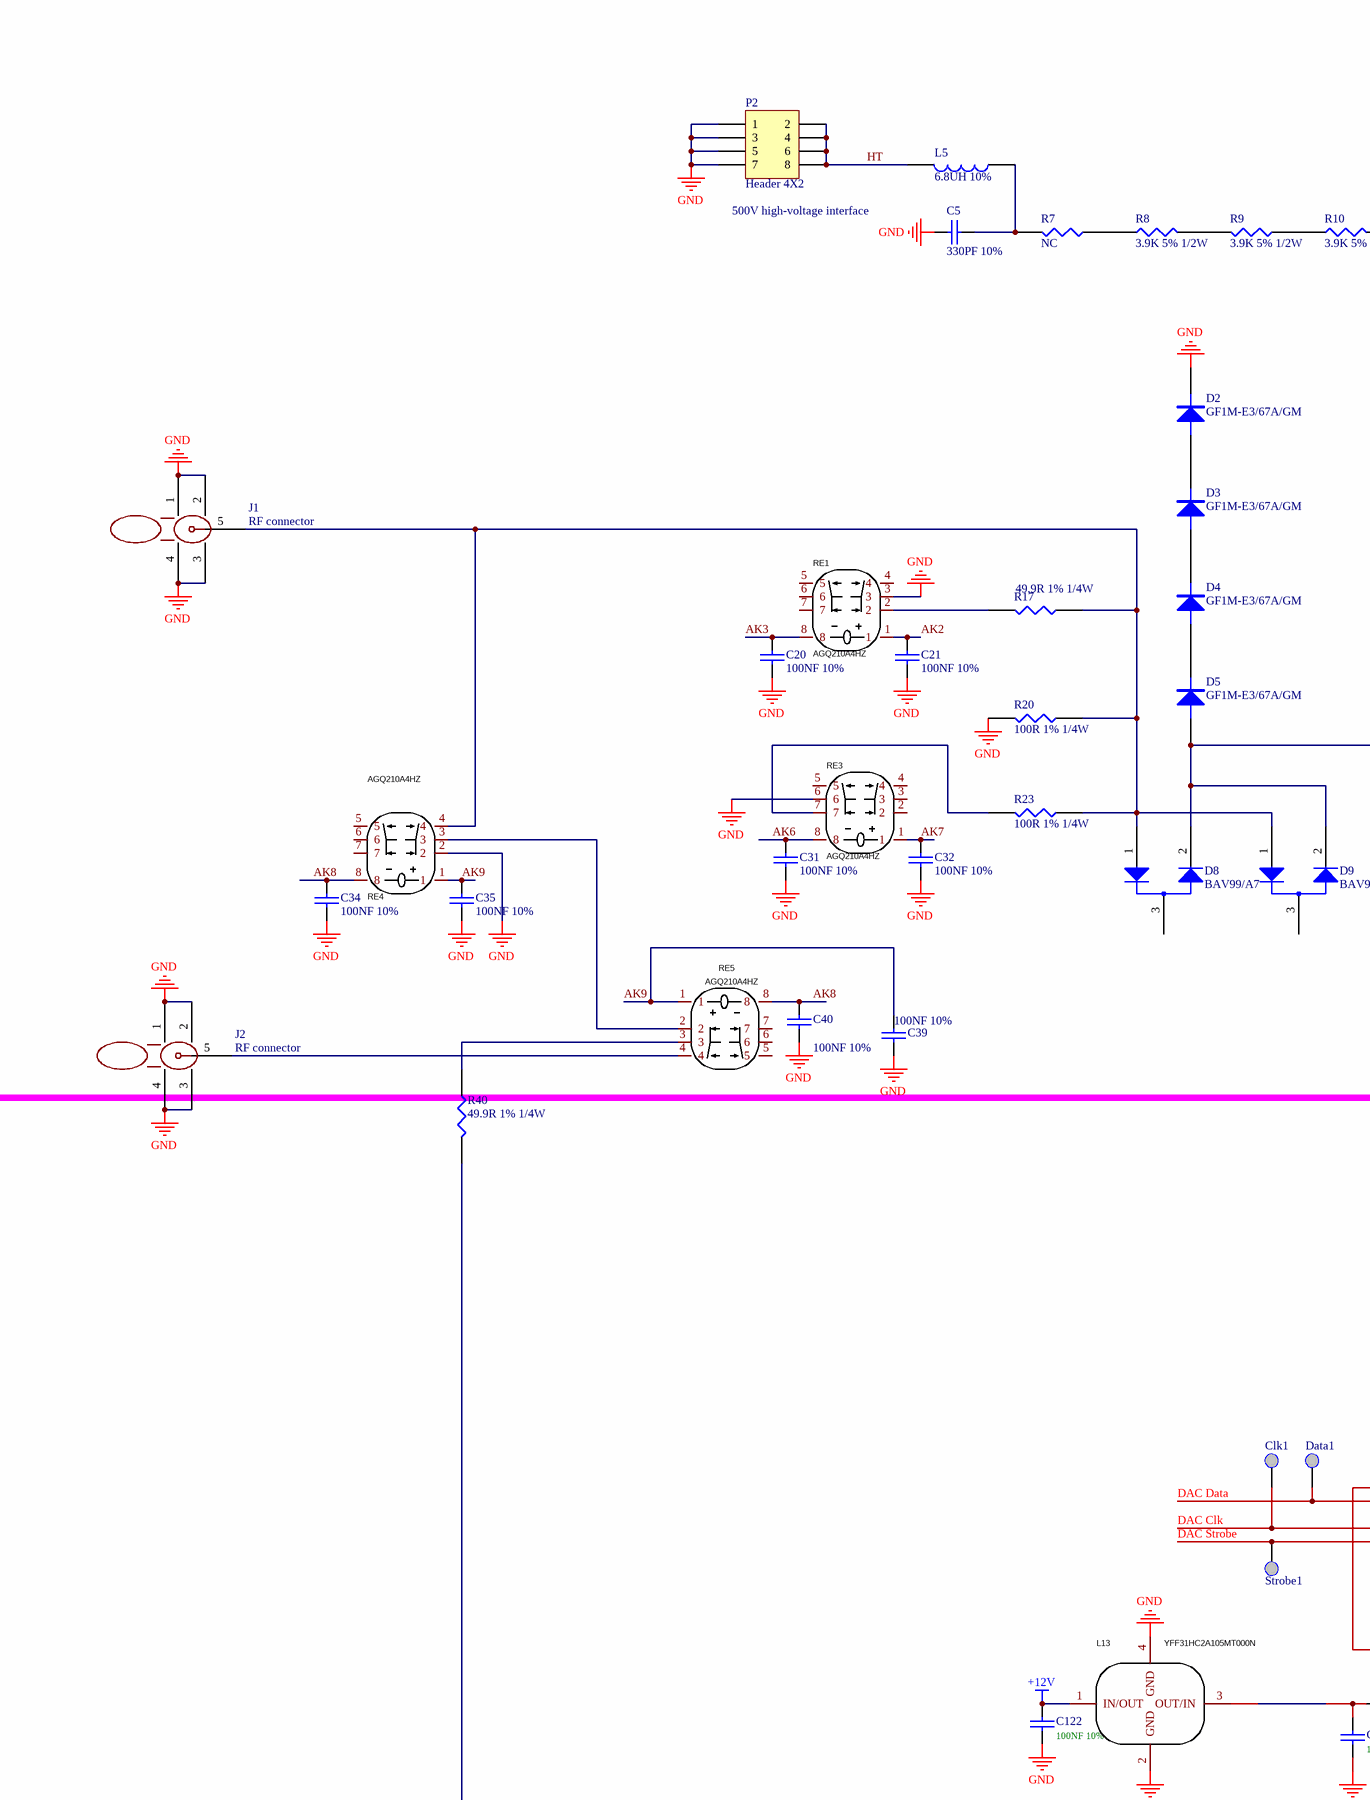
[diagram p0: PCBE109560-5.SchDoc, top left]
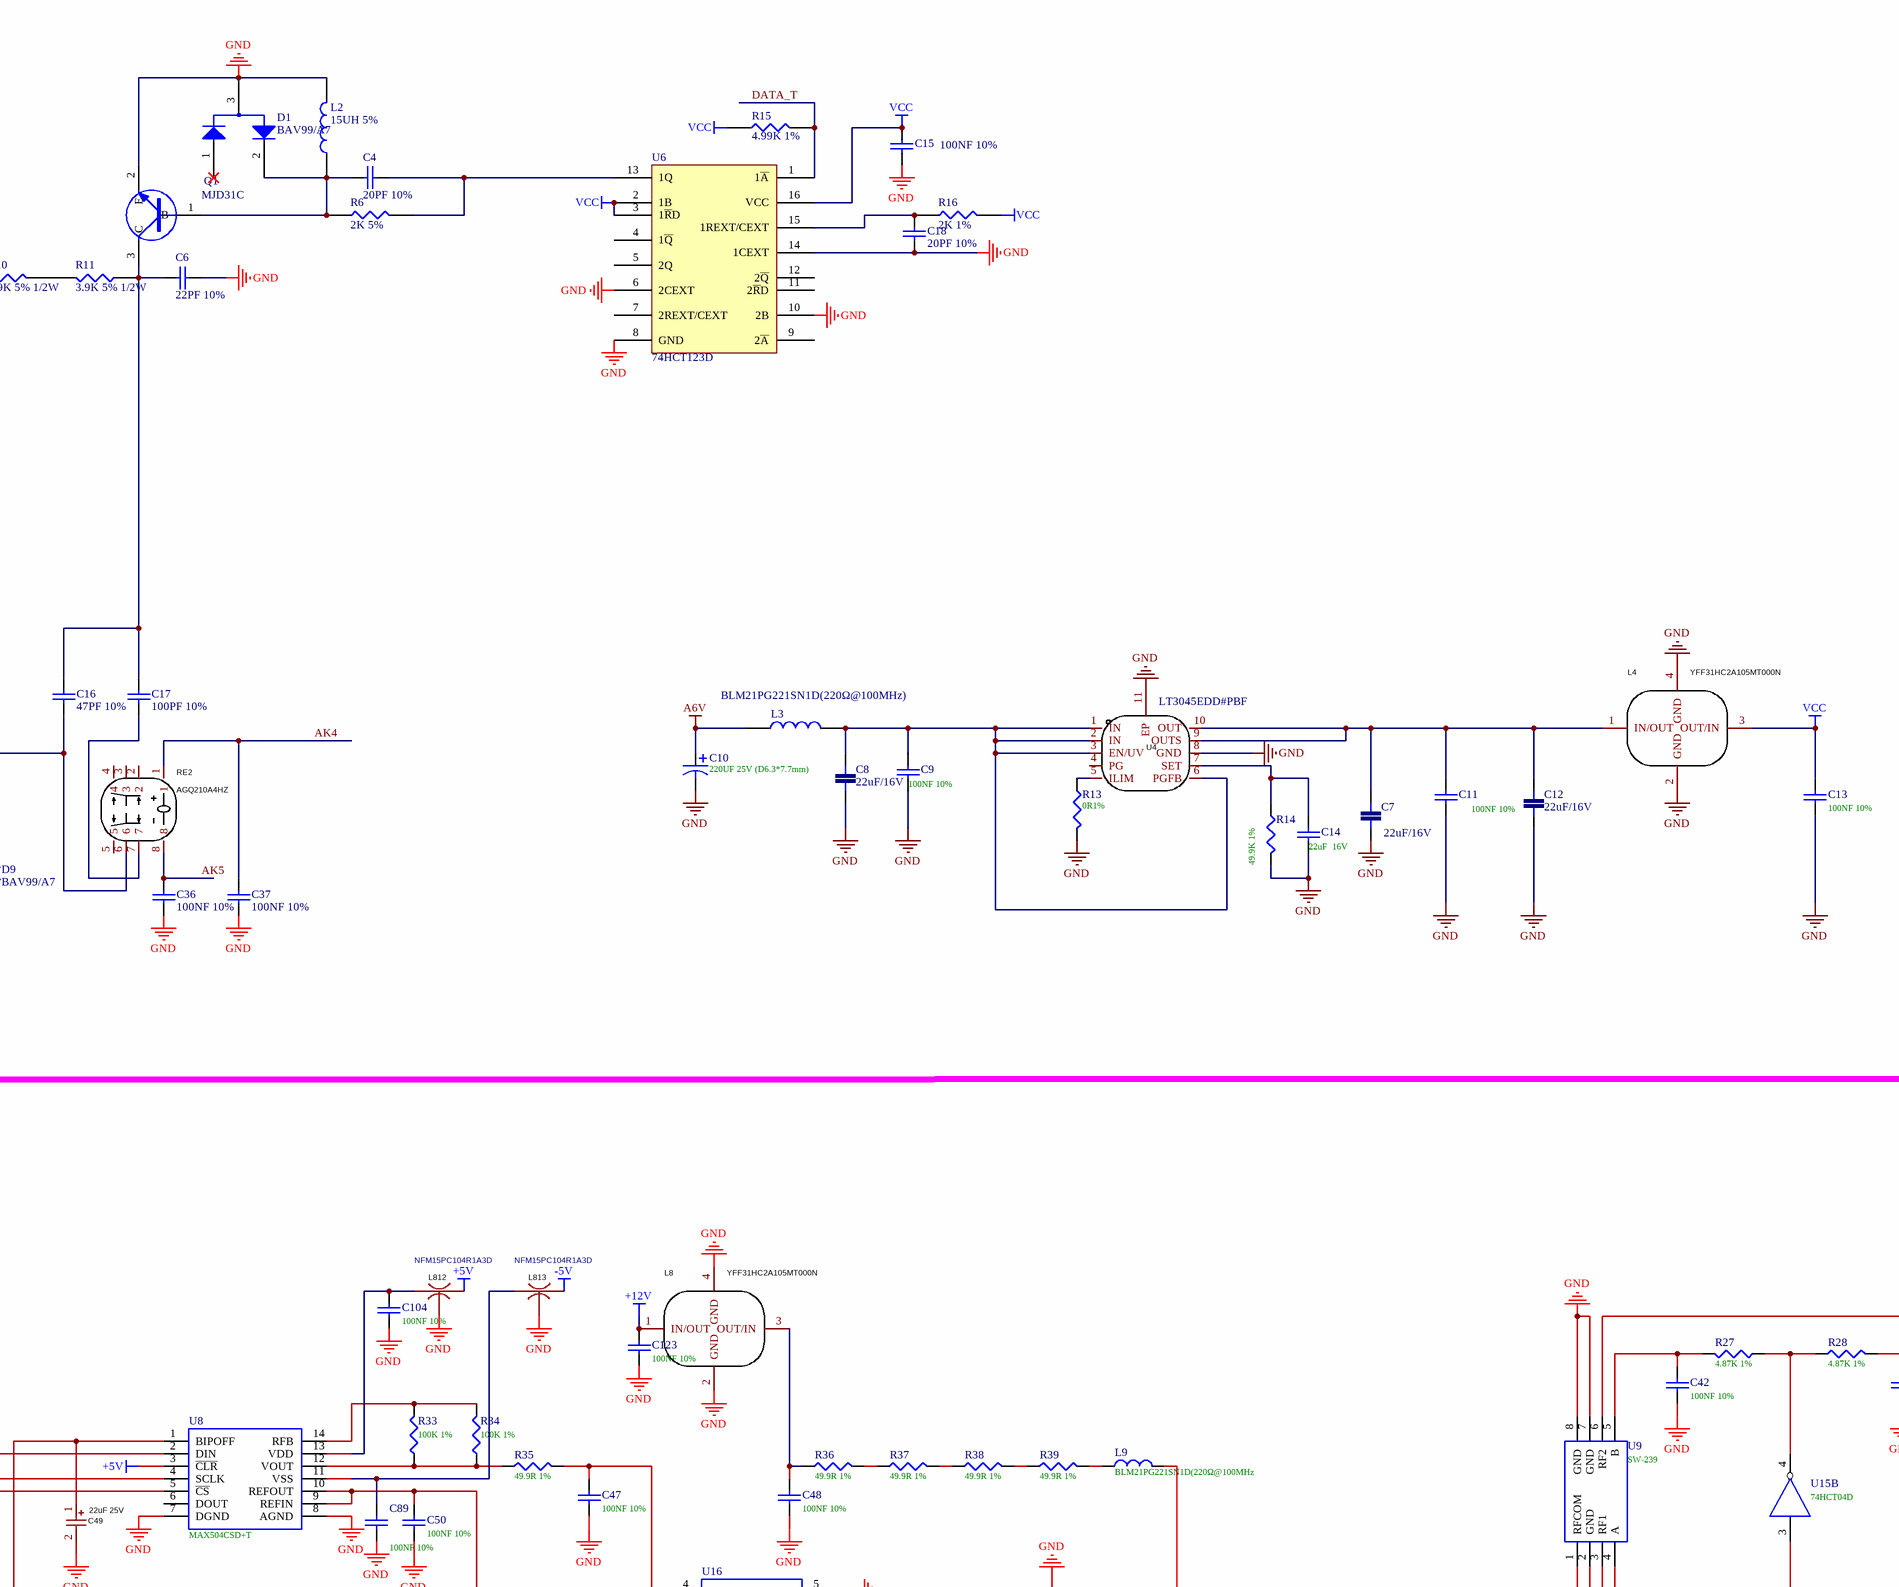
[diagram p1: PCBE109560-5.SchDoc, top middle]
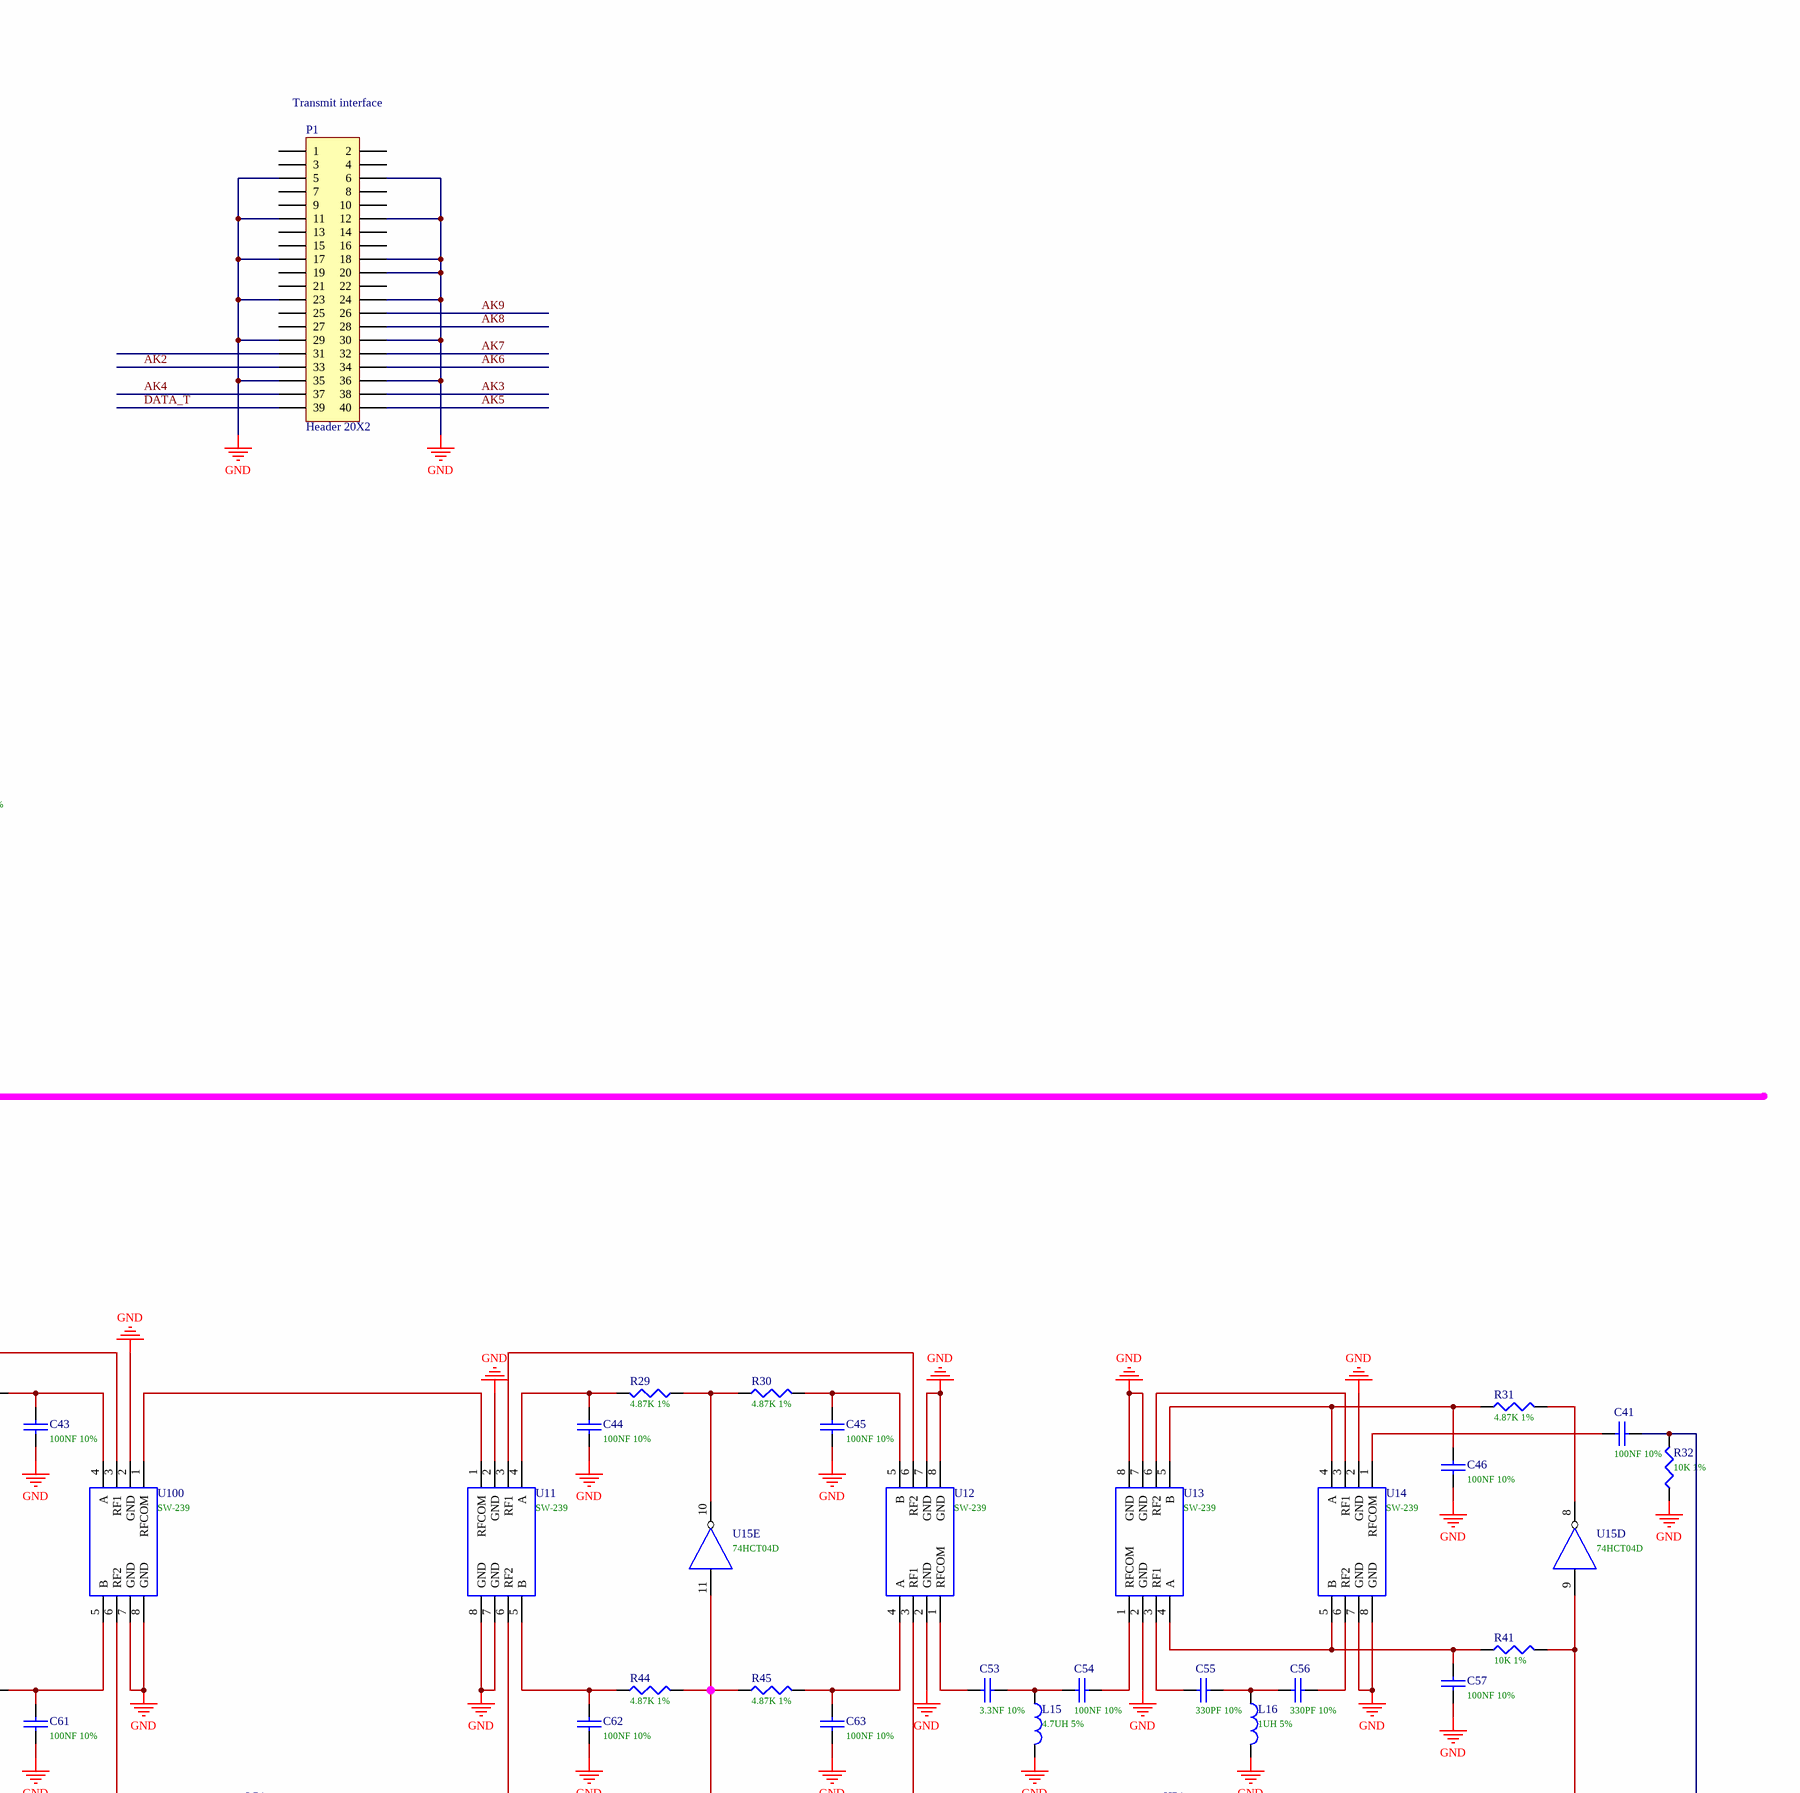
[diagram p2: PCBE109560-5.SchDoc, top right]
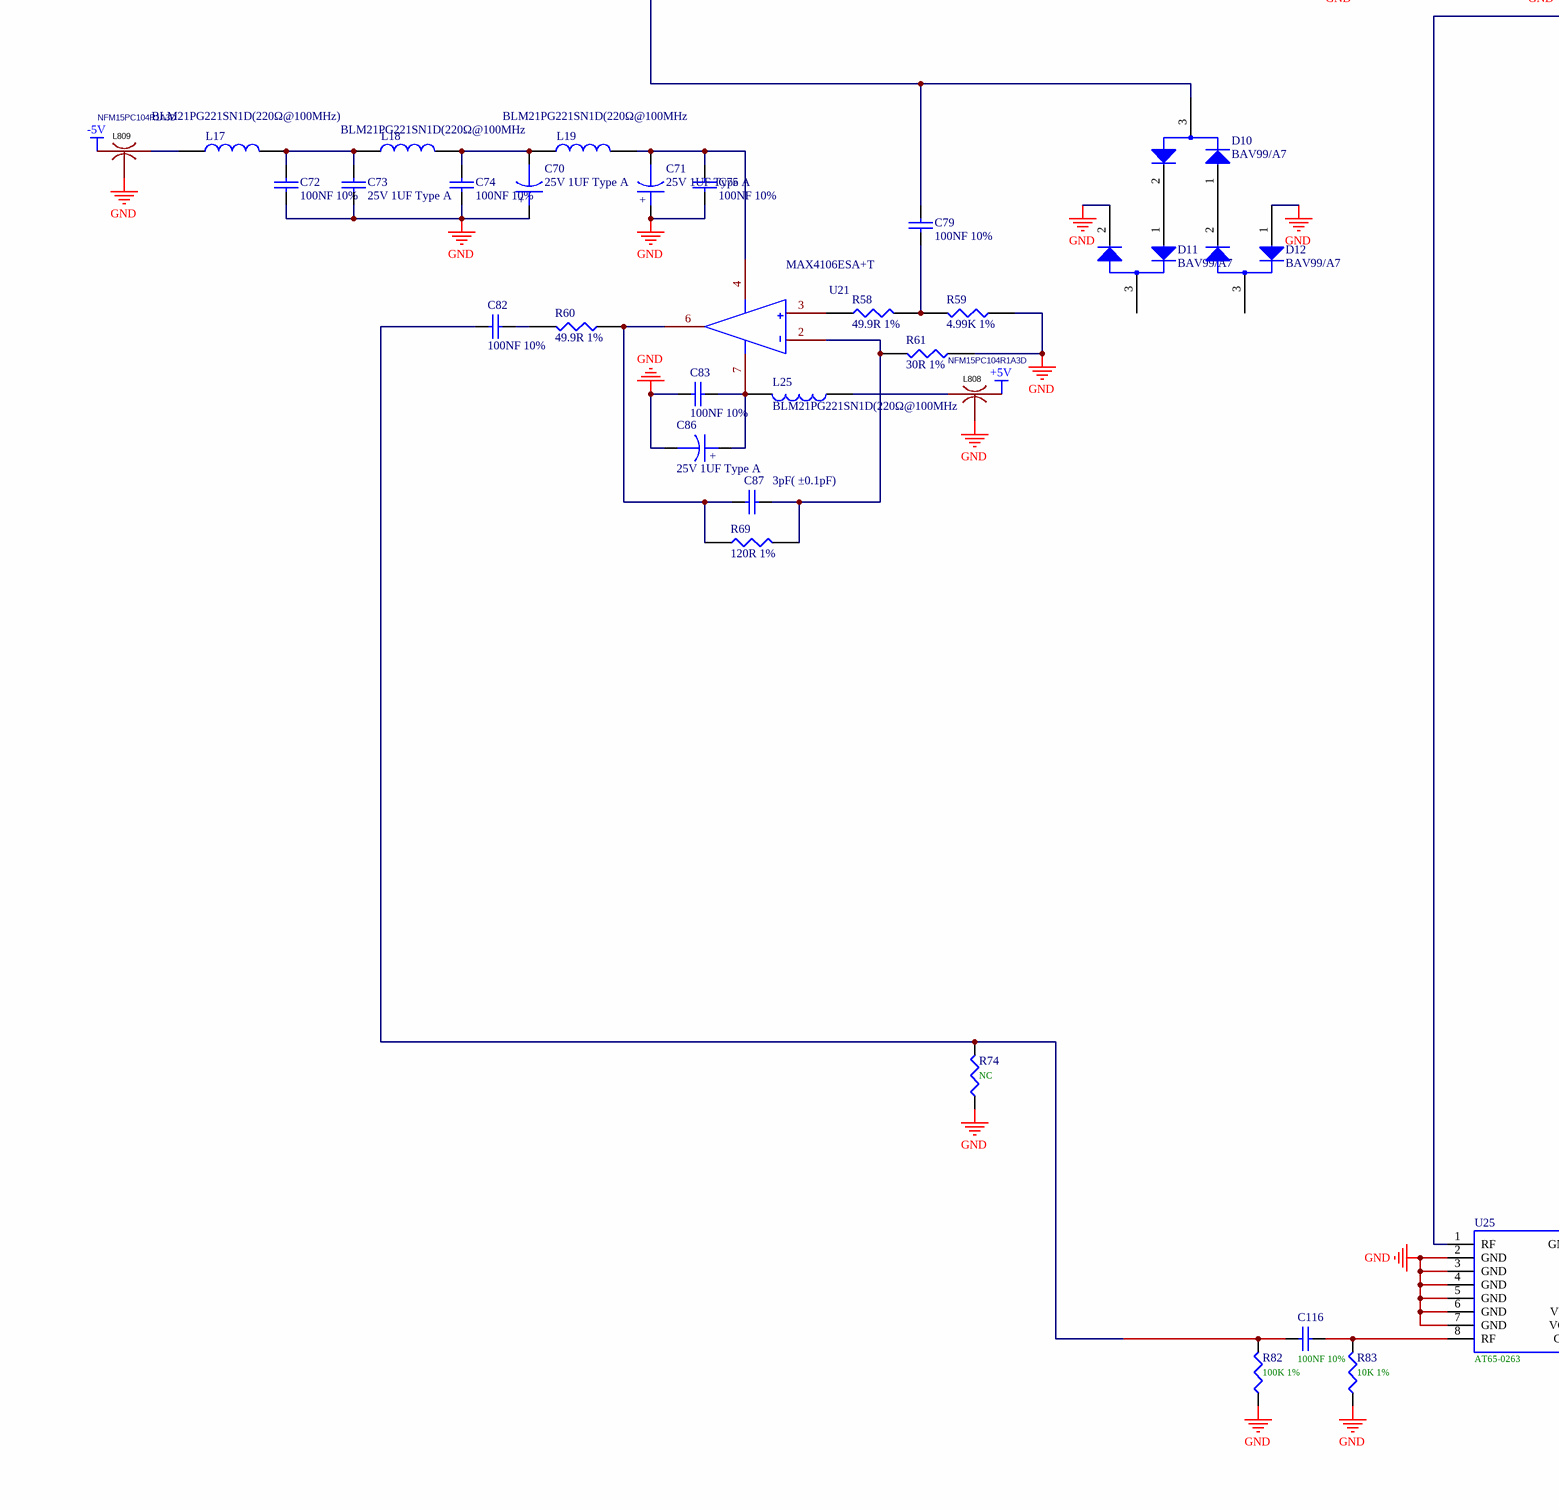
[diagram p3: PCBE109560-5.SchDoc, bottom left]
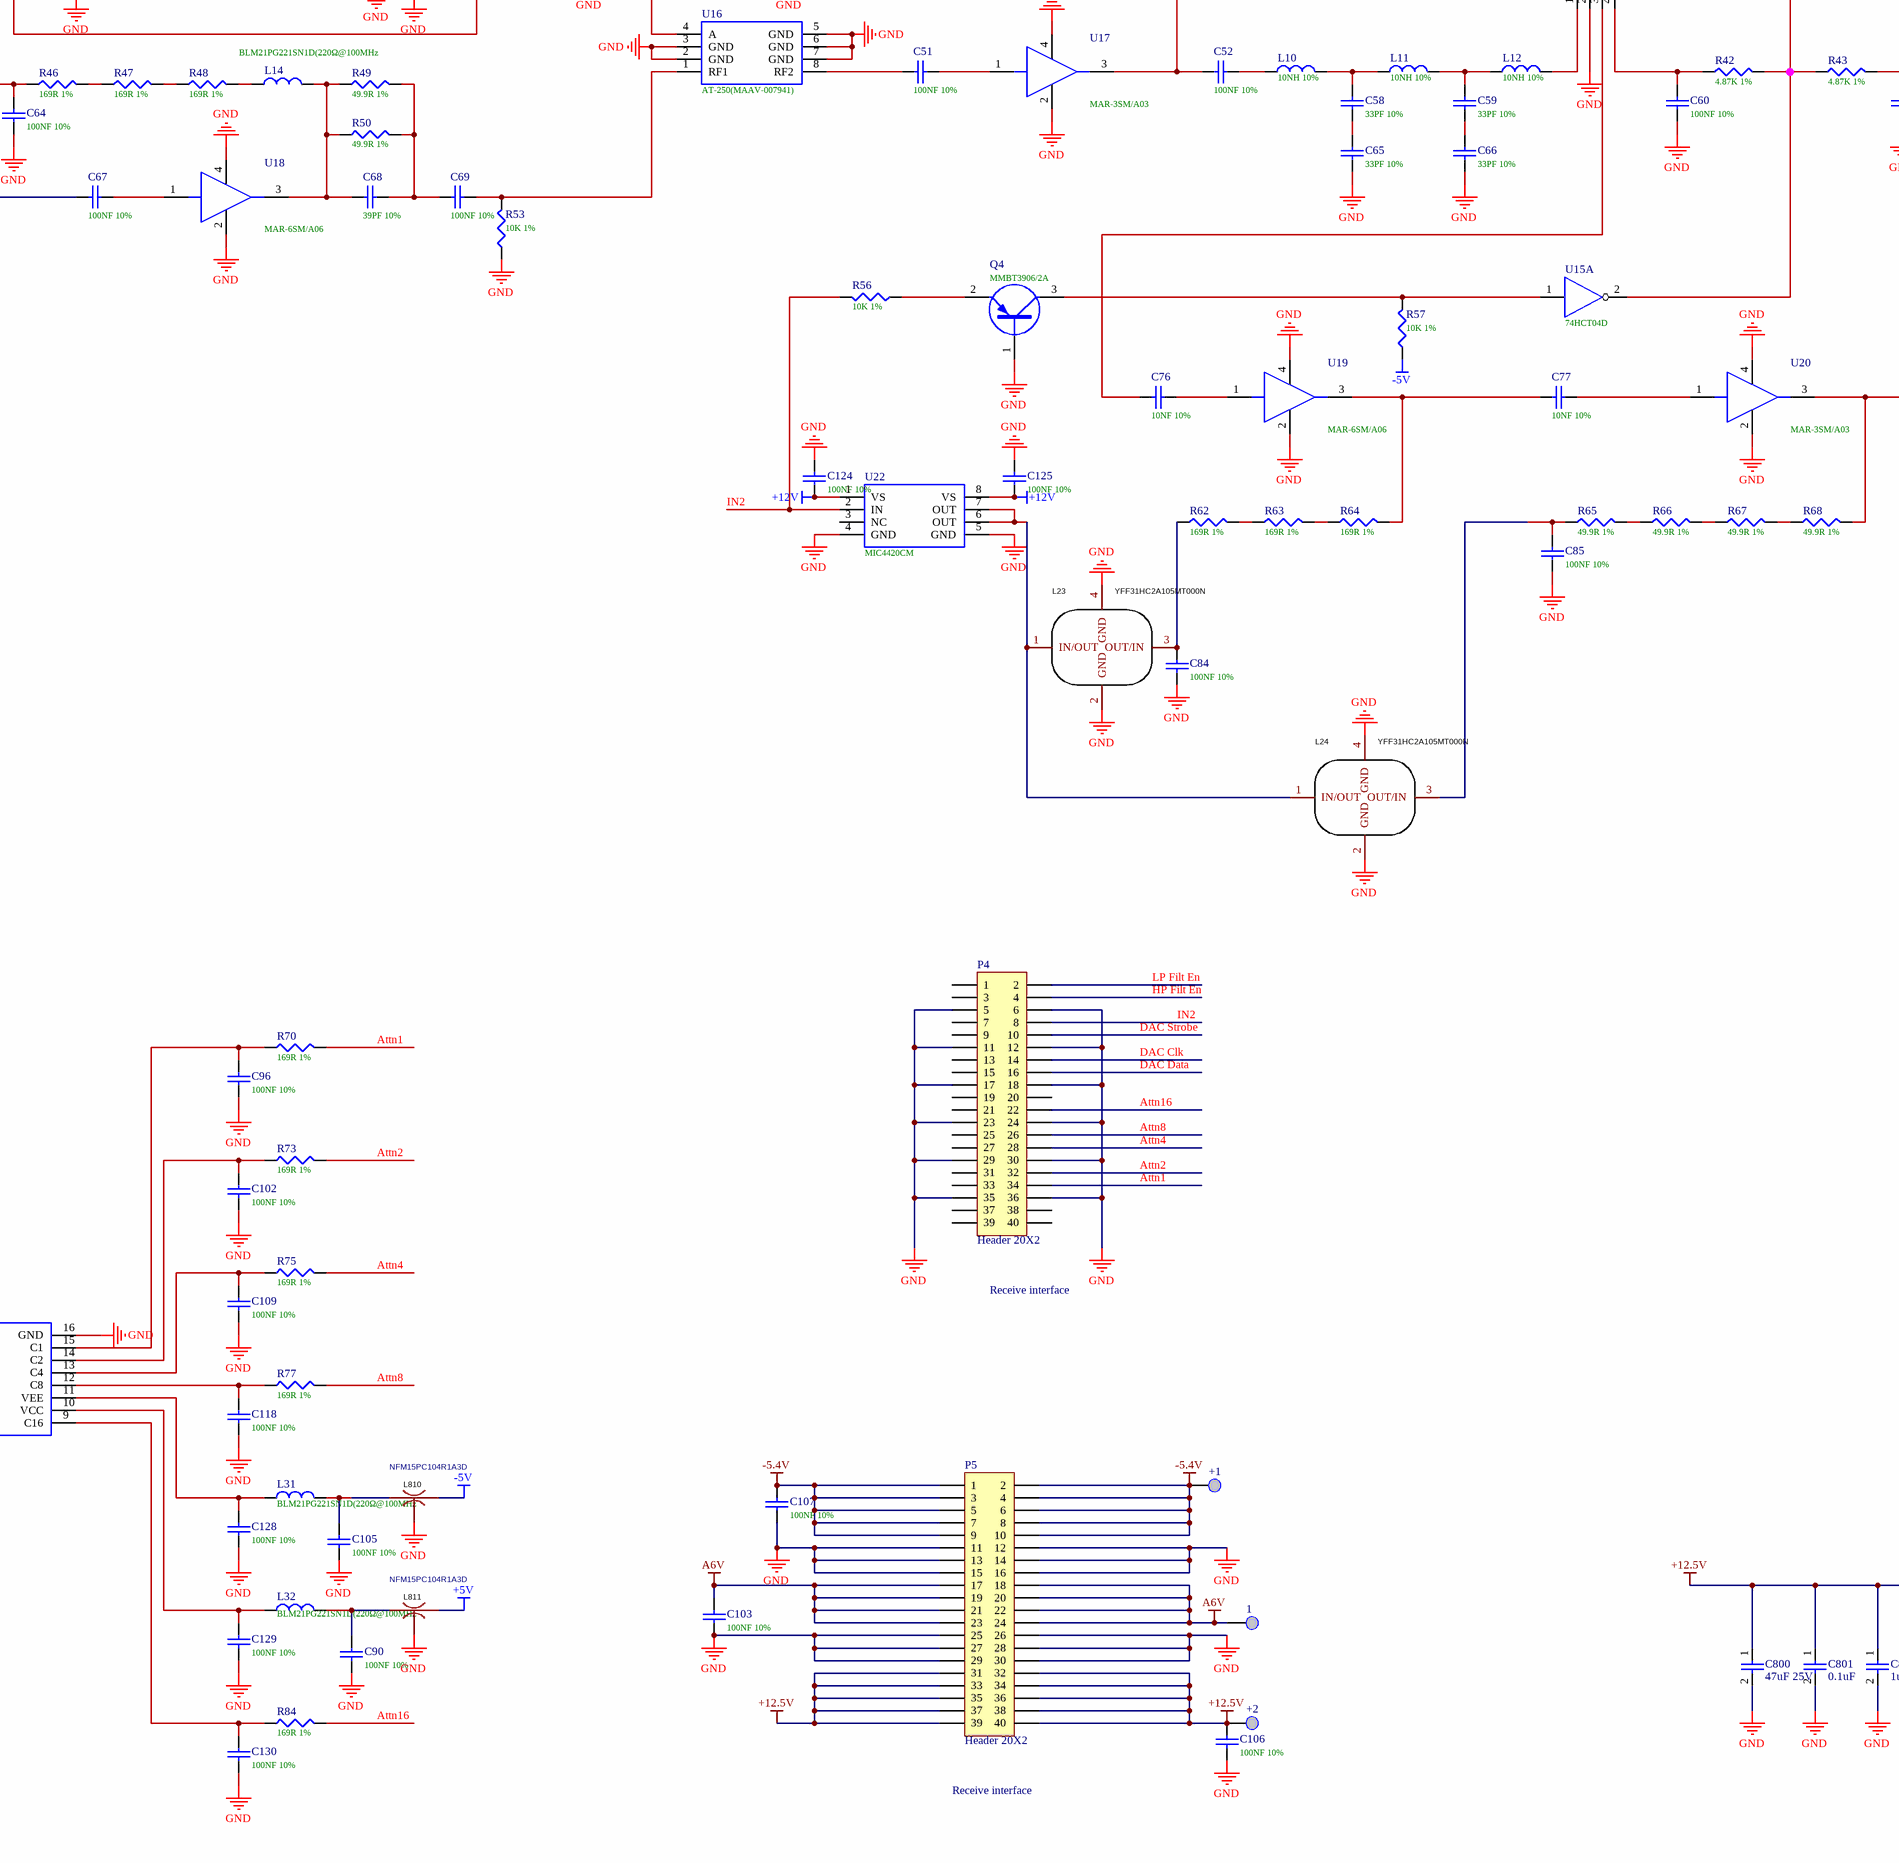
[diagram p4: PCBE109560-5.SchDoc, bottom middle]
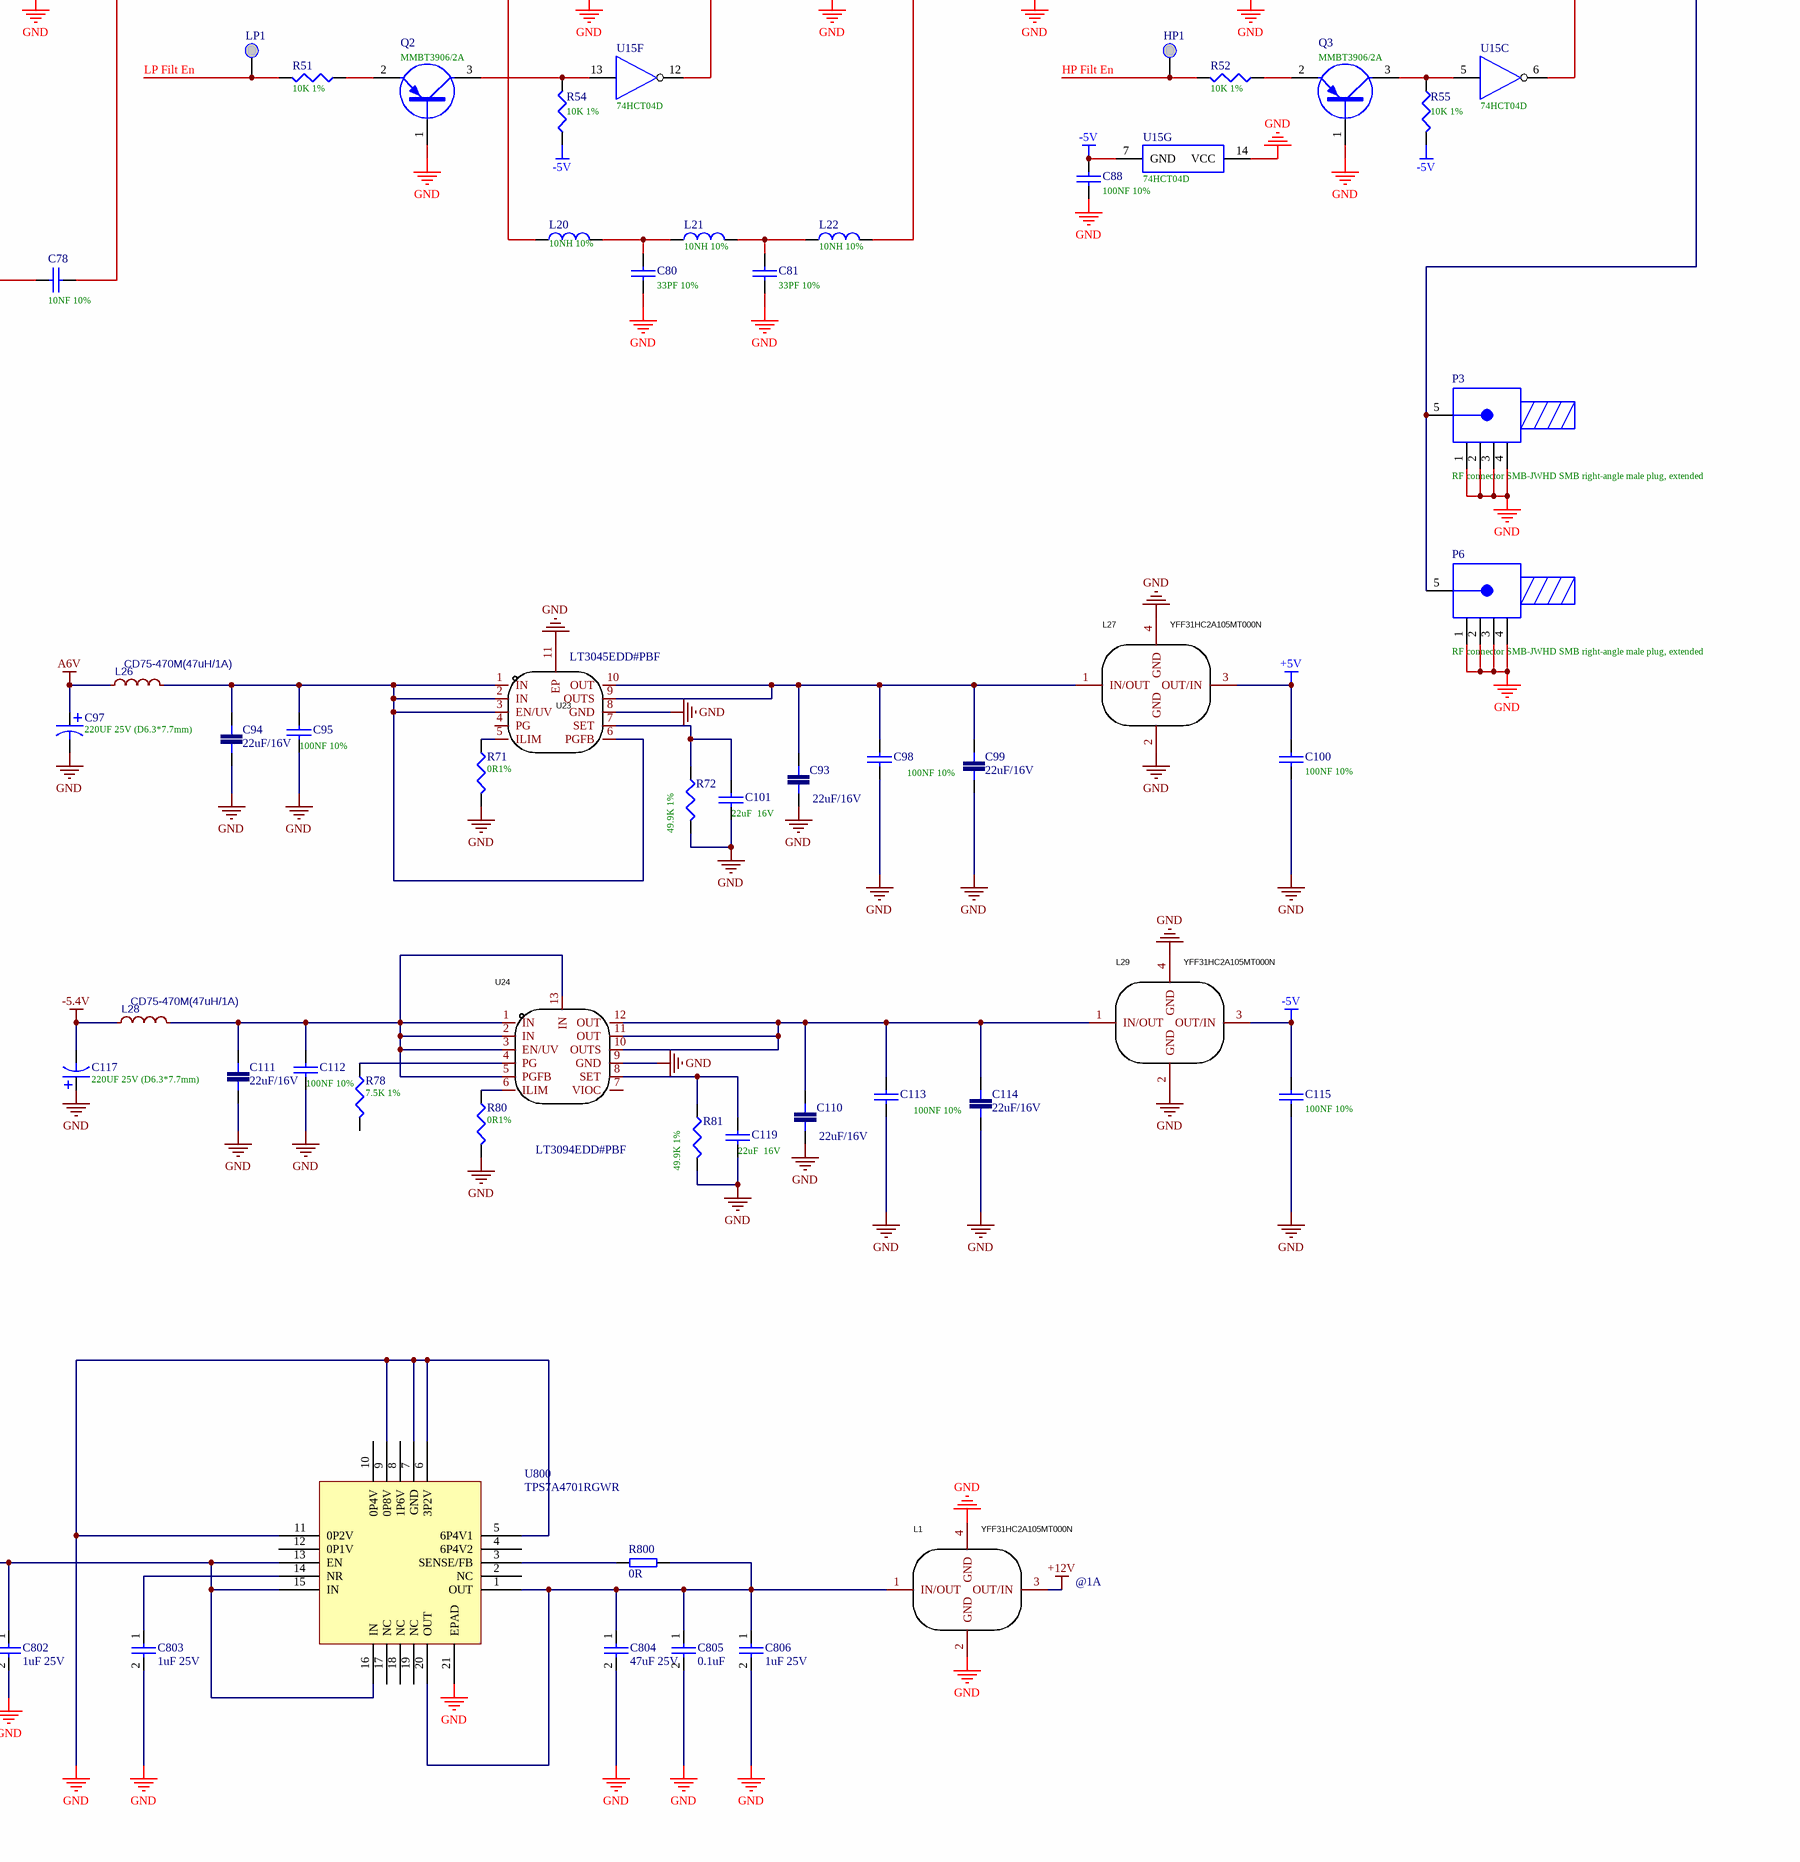
[diagram p5: PCBE109560-5.SchDoc, bottom right]
# Altium schematic sheet PCBE109560-5.SchDoc (part 1 of 2)
size E; SheetNumber: 0; SheetTotal: 0